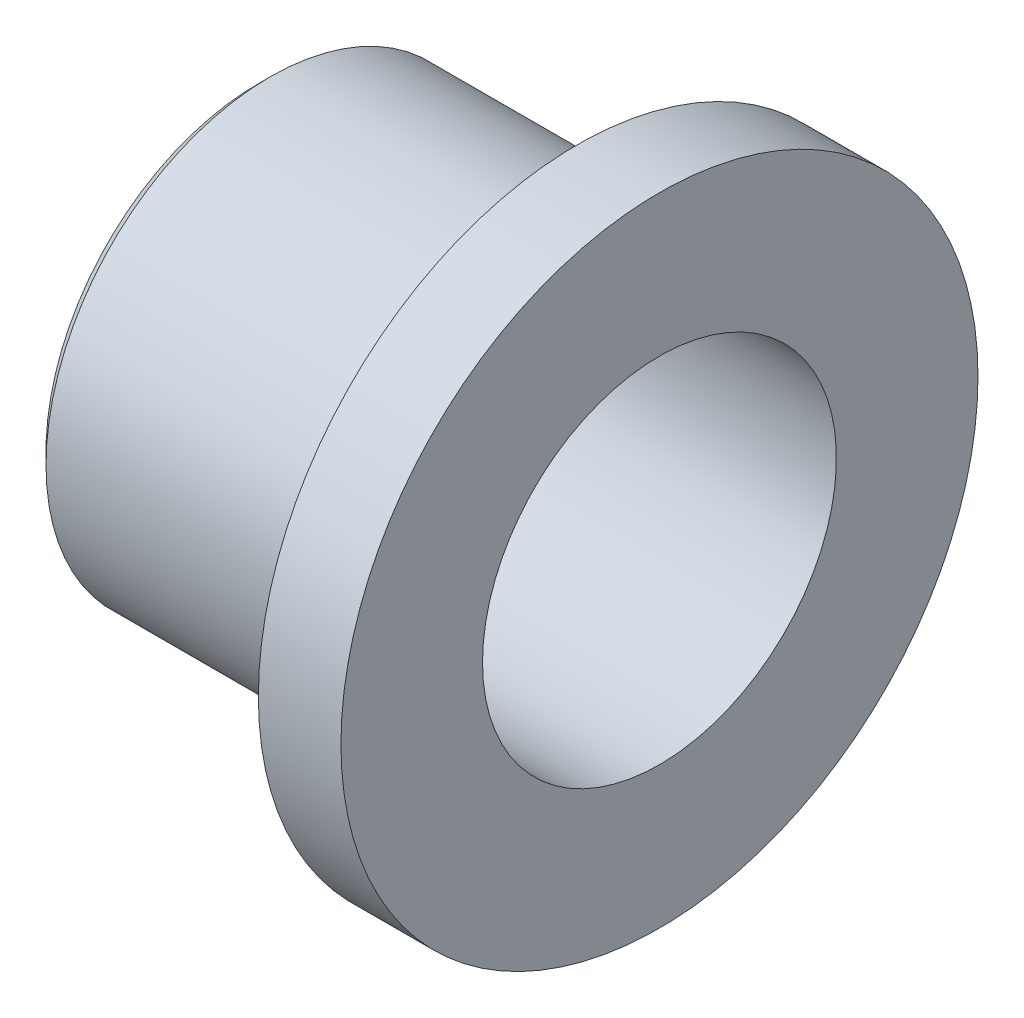
from build123d import *

# Parameters (mm, degrees)
CHAMFER1_SIZE = 1


with BuildPart() as part:
    # Sketch1 → Revolve1 (revolve)
    with BuildSketch(Plane.XY, mode=Mode.PRIVATE) as revolve1_sk:
        Polygon((0, 15), (34, 15), (34, 27), (27, 27), (27, 19), (0, 19), align=None)
    revolve(revolve1_sk.sketch.rotate(Axis((0, 0, 0), (1, 0, 0)), 90), axis=Axis((0, 0, 0), (1, 0, 0)))

    # Chamfer1
    chamfer1_edges = [part.edges().sort_by_distance(p)[0] for p in [
        (0, 0, -19),
    ]]
    chamfer(chamfer1_edges, length=CHAMFER1_SIZE)


solid = part.part
